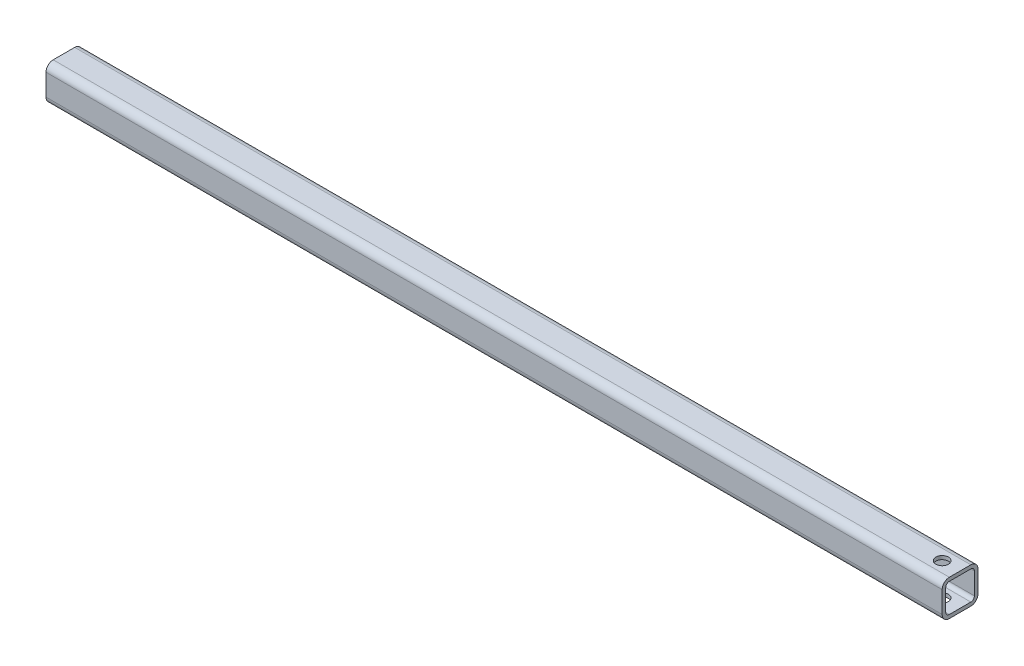
SolidWorks part; units mm, degrees
material "Q235A"
ref_plane "前视基准面" through (0, 0, 0) normal (0, 0, 1) x (1, 0, 0)
ref_plane "上视基准面" through (0, 0, 0) normal (0, 1, 0) x (1, 0, 0)
ref_plane "右视基准面" through (0, 0, 0) normal (1, 0, 0) x (0, 0, -1)
sketch "草图1" plane through (0, 0, 0) normal (0, 1, 0) x (1, 0, 0)
  line L0 (0, 0) -> (-1000, 0)
  dimension "D1" = 1000
other "Gb／6728-1986方形空心型钢 040 X 40 X 4(1)"
ref_plane "基准面1" through (0, 0, 0) normal (-1, 0, 0) x (0, 0, 1)
sketch "Sketch12" plane through (0, 0, 0) normal (-1, 0, 0) x (0, 0, 1)
  line L0 (-12, -16) -> (12, -16)
  line L1 (-16, -12) -> (-16, 12)
  line L2 (12, 16) -> (-12, 16)
  line L3 (16, 12) -> (16, -12)
  line L4 (-12, -20) -> (12, -20)
  line L5 (-20, -12) -> (-20, 12)
  line L6 (12, 20) -> (-12, 20)
  line L7 (20, 12) -> (20, -12)
  arc A0 (20, 12) -> (12, 20) centre (12, 12) ccw
  arc A1 (12, -20) -> (20, -12) centre (12, -12) ccw
  arc A2 (-20, -12) -> (-12, -20) centre (-12, -12) ccw
  arc A3 (-12, 20) -> (-20, 12) centre (-12, 12) ccw
  arc A4 (-12, 16) -> (-16, 12) centre (-12, 12) ccw
  arc A5 (16, 12) -> (12, 16) centre (12, 12) ccw
  arc A6 (12, -16) -> (16, -12) centre (12, -12) ccw
  arc A7 (-16, -12) -> (-12, -16) centre (-12, -12) ccw
  point P0 (-20, 0)
  point P1 (20, 0)
  point P2 (0, 20)
  point P3 (0, -20)
  point P4 (0, 0)
  point P5 (-20, -20)
  point P6 (20, -20)
  point P7 (20, 20)
  point P8 (-20, 20)
  point P33 (0, 0)
  dimension "D1" = 8
  dimension "Thickness" = 4
  dimension "V_leg" = 40
sketch "草图6" plane through (-1000, 0, 0) normal (-1, 0, 0) x (0, 0, 1)
  line L0 (16, -12) -> (16, 12) construction
  line L1 (-12, -16) -> (12, -16) construction
  line L2 (-16, 12) -> (-16, -12) construction
  line L3 (12, 16) -> (-12, 16) construction
  line L4 (16, -12) -> (16, 12)
  line L5 (-12, -16) -> (12, -16)
  line L6 (-16, 12) -> (-16, -12)
  line L7 (12, 16) -> (-12, 16)
  arc A0 (16, 12) -> (12, 16) centre (12, 12) ccw construction
  arc A1 (12, -16) -> (16, -12) centre (12, -12) ccw construction
  arc A2 (-16, -12) -> (-12, -16) centre (-12, -12) ccw construction
  arc A3 (-12, 16) -> (-16, 12) centre (-12, 12) ccw construction
  arc A4 (16, 12) -> (12, 16) centre (12, 12) ccw
  arc A5 (12, -16) -> (16, -12) centre (12, -12) ccw
  arc A6 (-16, -12) -> (-12, -16) centre (-12, -12) ccw
  arc A7 (-12, 16) -> (-16, 12) centre (-12, 12) ccw
extrude "凸台-拉伸1" [suppressed] add sketch "草图6" against normal blind 10 separate body
hole_wizard "M16 螺纹孔1" positions "草图9" profile "草图10" tap size "M16" standard "ISO" end condition through all
sketch "草图9" plane through (0, 20, 0) normal (0, 1, 0) x (1, 0, 0)
  point P0 (-20, 0)
  dimension "D1" = 20
sketch "草图10" plane through (-20, 20, 0) normal (1, 0, 0) x (0, 0, 1)
  line L0 (0, 0) -> (0, 40)
  line L1 (0, 40) -> (7, 40)
  line L2 (7, 40) -> (7, 0)
  line L5 (7, 0) -> (0, 0)
  line L11 (0, -6.35) -> (0, 107.95) construction
  dimension "通孔螺纹孔钻头直径" = 14
  dimension "通孔螺纹孔钻头深度" = 40
cosmetic thread "孔螺蚊线1" parameters "D2"=16
